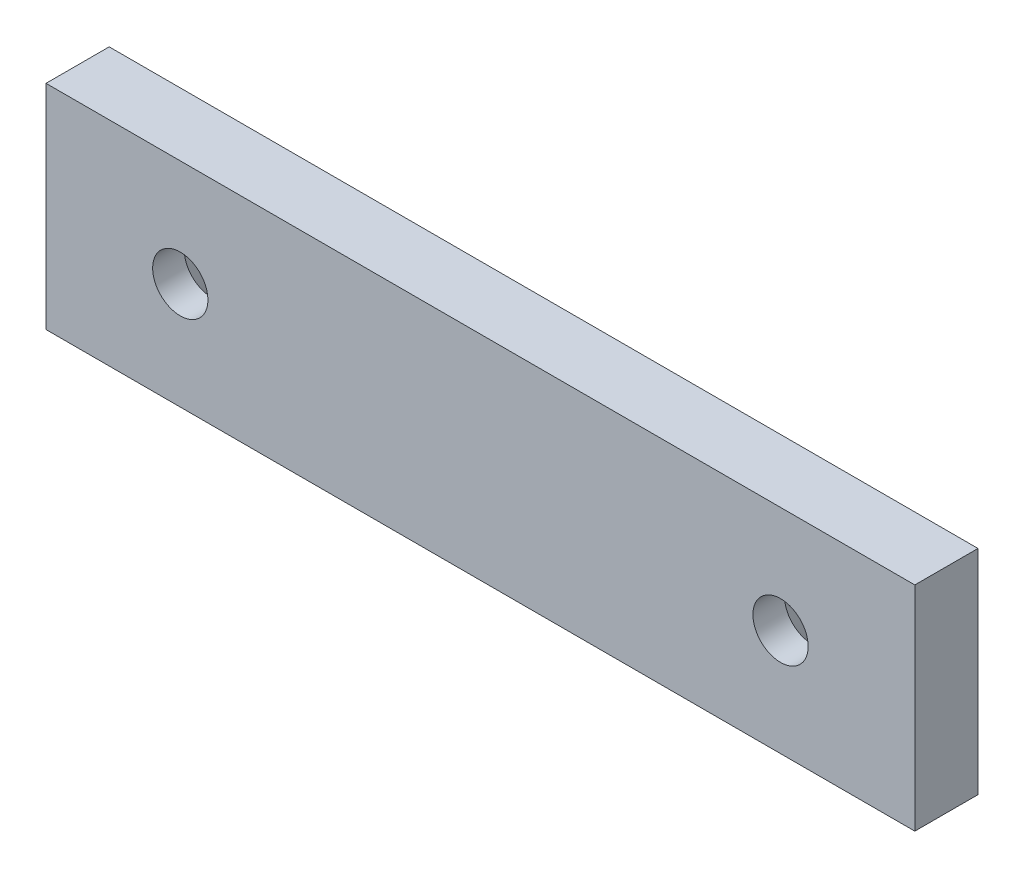
SolidWorks part; units mm, degrees
ref_plane "Front Plane" through (0, 0, 0) normal (0, 0, 1) x (1, 0, 0)
ref_plane "Top Plane" through (0, 0, 0) normal (0, 1, 0) x (1, 0, 0)
ref_plane "Right Plane" through (0, 0, 0) normal (1, 0, 0) x (0, 0, -1)
sketch "Sketch1" plane through (0, 0, 0) normal (0, 0, 1) x (1, 0, 0)
  line L2 (-55, -13.5) -> (55, -13.5)
  line L3 (-55, -13.5) -> (-55, 13.5)
  line L4 (-55, 13.5) -> (55, 13.5)
  line L5 (55, -13.5) -> (55, 13.5)
  line L6 (-55, -13.5) -> (55, 13.5) construction
  line L7 (-55, 13.5) -> (55, -13.5) construction
  point P1 (0, 0)
  dimension "D1" = 110
  dimension "D2" = 27
extrude "Boss-Extrude1" add sketch "Sketch1" along normal blind 8
sketch "Sketch2" plane through (0, 0, 0) normal (0, 1, 0) x (1, 0, 0)
  line L0 (-38, 0) -> (-38, -8) construction
  line L1 (55, 0) -> (-55, 0) construction
  line L2 (55, -8) -> (-55, -8) construction
  line L3 (-30.5, 0) -> (-34.5, -4)
  line L4 (-34.5, -4) -> (-34.5, -8)
  line L5 (-34.5, -8) -> (-38, -8)
  line L6 (-30.5, 0) -> (-38, 0)
  line L7 (-38, 0) -> (-38, -8)
  dimension "D1" = 45
  dimension "D2" = 3.5
  dimension "D3" = 38
  dimension "D4" = 7.5
revolve "Cut-Revolve2" cut sketch "Sketch2" angle 360 about L0
mirror "Mirror1" about plane through (0, 0, 0) normal (1, 0, 0) of "Cut-Revolve2"
